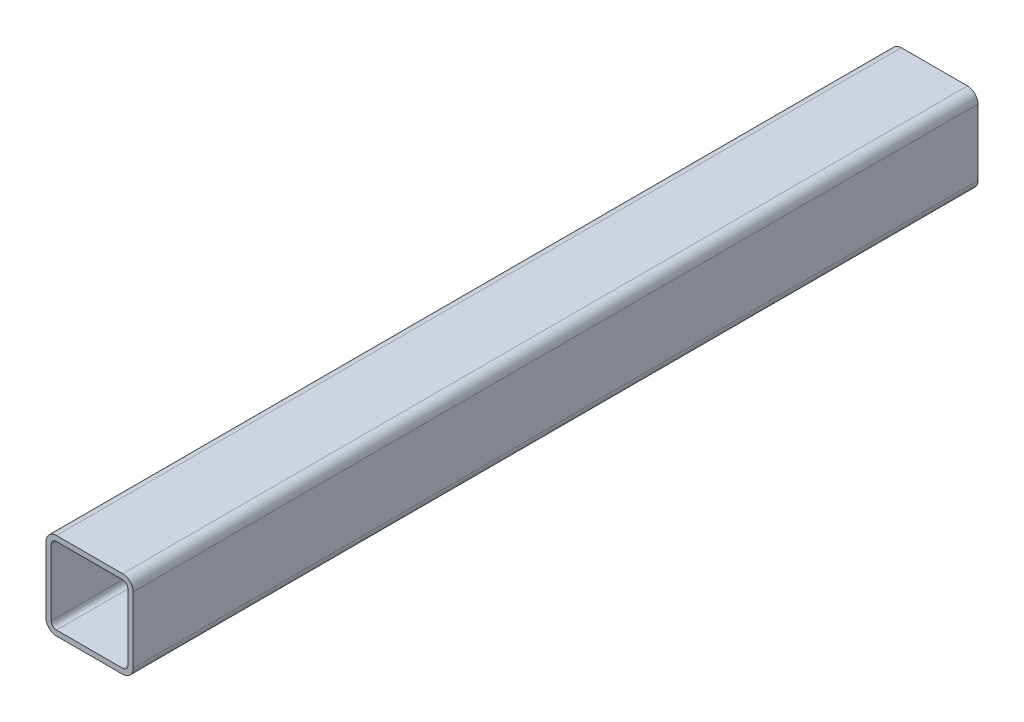
SolidWorks part; units mm, degrees
material "Q235B"
ref_plane "前视基准面" through (0, 0, 0) normal (0, 0, 1) x (1, 0, 0)
ref_plane "上视基准面" through (0, 0, 0) normal (0, 1, 0) x (1, 0, 0)
ref_plane "右视基准面" through (0, 0, 0) normal (1, 0, 0) x (0, 0, -1)
other "Configuration Table"
sketch "草图1" plane through (0, 0, 0) normal (1, 0, 0) x (0, 0, -1)
  line L0 (-242.5, 0) -> (242.5, 0)
other "Gb／6728-1986方形空心型钢 050 X 50 X 3(1)"
ref_plane "基准面1" through (0, 0, 242.5) normal (0, 0, -1) x (0, 1, 0)
sketch "Sketch1" plane through (0, 0, 242.5) normal (0, 0, -1) x (0, 1, 0)
  line L0 (-19, -22) -> (19, -22)
  line L1 (-22, -19) -> (-22, 19)
  line L2 (19, 22) -> (-19, 22)
  line L3 (22, 19) -> (22, -19)
  line L4 (-19, -25) -> (19, -25)
  line L5 (-25, -19) -> (-25, 19)
  line L6 (19, 25) -> (-19, 25)
  line L7 (25, 19) -> (25, -19)
  arc A0 (25, 19) -> (19, 25) centre (19, 19) ccw
  arc A1 (19, -25) -> (25, -19) centre (19, -19) ccw
  arc A2 (-25, -19) -> (-19, -25) centre (-19, -19) ccw
  arc A3 (-19, 25) -> (-25, 19) centre (-19, 19) ccw
  arc A4 (-19, 22) -> (-22, 19) centre (-19, 19) ccw
  arc A5 (22, 19) -> (19, 22) centre (19, 19) ccw
  arc A6 (19, -22) -> (22, -19) centre (19, -19) ccw
  arc A7 (-22, -19) -> (-19, -22) centre (-19, -19) ccw
  point P0 (-25, 0)
  point P1 (25, 0)
  point P2 (0, 25)
  point P3 (0, -25)
  point P4 (0, 0)
  point P5 (-25, -25)
  point P6 (25, -25)
  point P7 (25, 25)
  point P8 (-25, 25)
  point P33 (0, 0)
  dimension "D1" = 6
  dimension "Thickness" = 3
  dimension "V_leg" = 50
equation "\"D2@草图1\"=\"D1@草图1\"/2"
